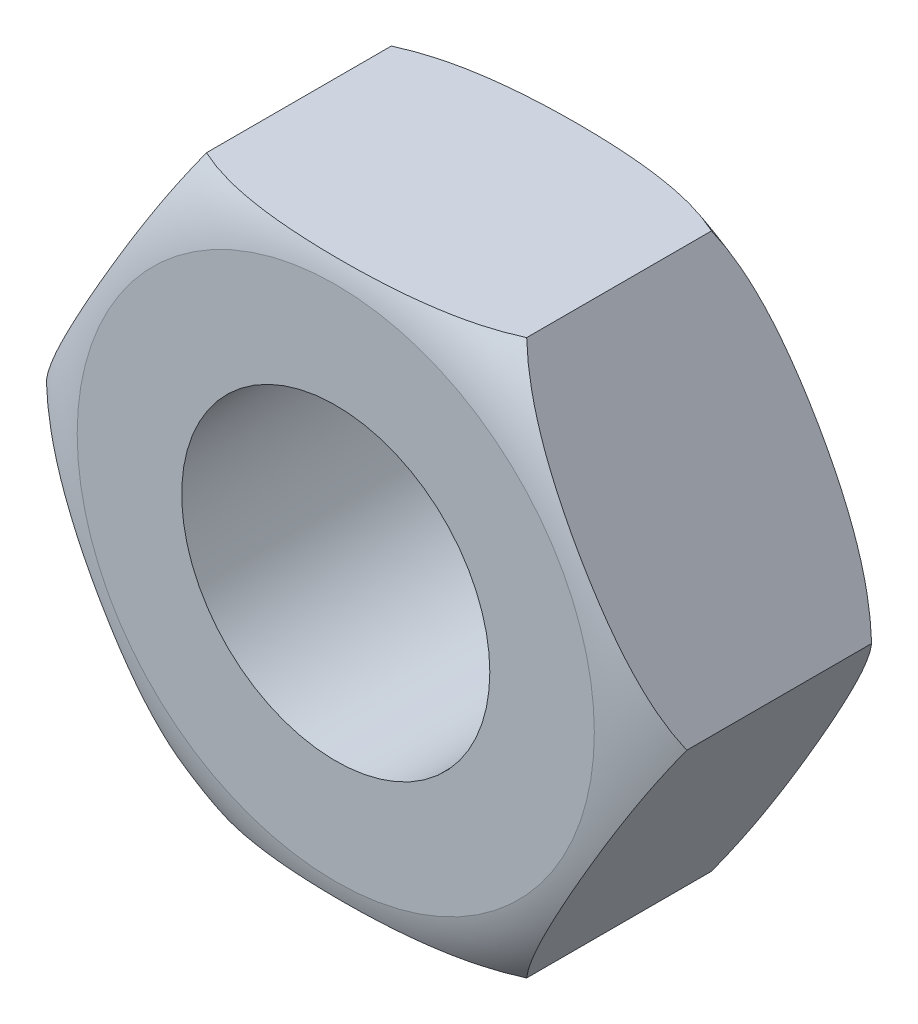
from build123d import *

# Parameters (mm, degrees)
SKETCH5_R           = 5
BOSS_EXTRUDE2_DEPTH = 8
SCALE_1_SCALE       = 1.875


with BuildPart() as part:
    # Sketch5 → Boss-Extrude2 (new body)
    with BuildSketch(Plane.XY):
        Polygon((10.392304845, 0), (5.196152423, 9), (-5.196152423, 9), (-10.392304845, 0), (-5.196152423, -9), (5.196152423, -9), align=None)
        Circle(SKETCH5_R, mode=Mode.SUBTRACT)
    extrude(amount=BOSS_EXTRUDE2_DEPTH)

    # Sketch6 → Cut-Revolve2 (revolve, cut)
    with BuildSketch(Plane(origin=(0, 0, 0), x_dir=(1, 0, 0), z_dir=(0, 1, 0))):
        with BuildLine():
            Line((-10.392304845, 0), (-10.392304845, -1))
            ThreePointArc((-10.392304845, -1), (-9.463602824, -0.357404043), (-8.392304845, 0))
            Line((-8.392304845, 0), (-10.392304845, 0))
        make_face()
        with BuildLine():
            Line((-10.392304845, -8), (-8.392304845, -8))
            ThreePointArc((-8.392304845, -8), (-9.463602824, -7.642595957), (-10.392304845, -7))
            Line((-10.392304845, -7), (-10.392304845, -8))
        make_face()
    revolve(axis=Axis((0, 0, 0), (0, 0, 1)), mode=Mode.SUBTRACT)


with BuildPart() as part_1:
    # Scale 1: scaled about (-5.25e-07, 1.59e-07, 3.999997472)
    add(part.part.scale(SCALE_1_SCALE).moved(Location((4.59e-07, -1.39e-07, -3.499997788))))


solid = part_1.part
